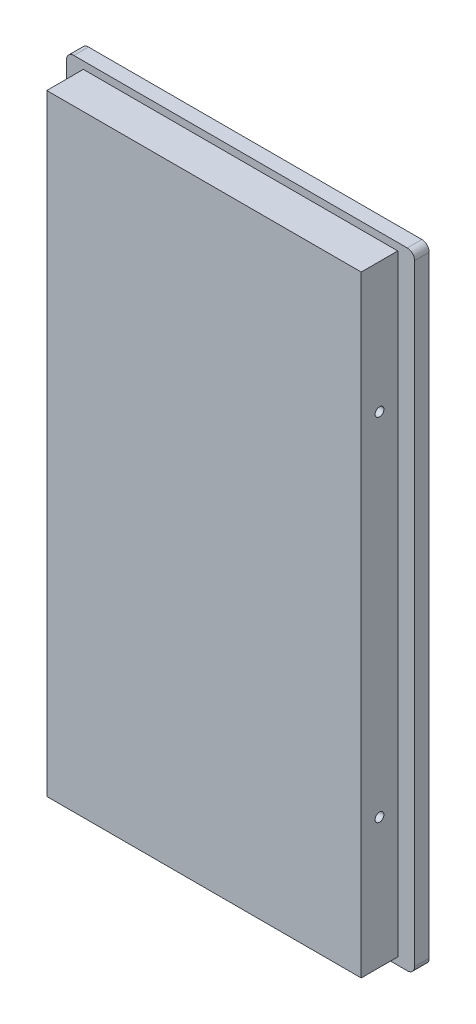
from build123d import *

# Parameters (mm, degrees)
EXTRUDE_1_DEPTH          = 10
SKETCH_2_W               = 215
SKETCH_2_H               = 418
EXTRUDE_2_DEPTH          = 25
CUT_EXTRUDE_1_DEPTH      = 314.565383931
CUT_EXTRUDE_1_DEPTH_BACK = 314.565383931
SKETCH_3_R               = 3
SKETCH_4_R               = 12.5
SKETCH_4_W               = 100
SKETCH_4_H               = 60
CUT_EXTRUDE_2_DEPTH      = 1


with BuildPart() as part:
    # 草图1 → 凸台-拉伸1 (new body)
    with BuildSketch(Plane.XY):
        with BuildLine():
            Line((-114, 214), (114, 214))
            ThreePointArc((114, 214), (117.535533906, 212.535533906), (119, 209))
            Line((119, 209), (119, -209))
            ThreePointArc((119, -209), (117.535533906, -212.535533906), (114, -214))
            Line((114, -214), (-114, -214))
            ThreePointArc((-114, -214), (-117.535533906, -212.535533906), (-119, -209))
            Line((-119, -209), (-119, 209))
            ThreePointArc((-119, 209), (-117.535533906, 212.535533906), (-114, 214))
        make_face()
    extrude(amount=EXTRUDE_1_DEPTH)

    # 草图2 → 凸台-拉伸2 (add)
    with BuildSketch(Plane.XY.offset(10)):
        Rectangle(SKETCH_2_W, SKETCH_2_H)
    extrude(amount=EXTRUDE_2_DEPTH)

    # 草图3 → 切除-拉伸1 (cut, two sides: drawn at the far end of the back side and taken through both)
    with BuildSketch(Plane(origin=(107.5, 0, 0), x_dir=(0, 0, -1), z_dir=(1, 0, 0)).offset(-CUT_EXTRUDE_1_DEPTH_BACK)):
        with Locations(Location((-22.5, 120, 0), (0, 0, 90))):
            Circle(SKETCH_3_R)
        with Locations(Location((-22.5, -120, 0), (0, 0, 90))):
            Circle(SKETCH_3_R)
    extrude(amount=CUT_EXTRUDE_1_DEPTH + CUT_EXTRUDE_1_DEPTH_BACK, mode=Mode.SUBTRACT)

    # 草图4 → 切除-拉伸2 (cut)
    with BuildSketch(Plane(origin=(0, 0, 0), x_dir=(-1, 0, 0), z_dir=(0, 0, -1))):
        with Locations((0, -26)):
            Circle(SKETCH_4_R)
        with Locations((60, -26)):
            Circle(SKETCH_4_R)
        with Locations((60, -86)):
            Circle(SKETCH_4_R)
        with Locations((60, -146)):
            Circle(SKETCH_4_R)
        with Locations((0, -86)):
            Circle(SKETCH_4_R)
        with Locations((0, -146)):
            Circle(SKETCH_4_R)
        with Locations(Location((-60, -146, 0), (0, 0, 180))):
            Circle(SKETCH_4_R)
        with Locations(Location((-60, -86, 0), (0, 0, 180))):
            Circle(SKETCH_4_R)
        with Locations(Location((-60, -26, 0), (0, 0, 180))):
            Circle(SKETCH_4_R)
        with Locations((0, 134)):
            Rectangle(SKETCH_4_W, SKETCH_4_H)
        with BuildLine():
            Line((-12.5, 36), (12.5, 36))
            ThreePointArc((12.5, 36), (14.5, 34), (12.5, 32))
            Line((12.5, 32), (-12.5, 32))
            ThreePointArc((-12.5, 32), (-14.5, 34), (-12.5, 36))
        make_face()
        with BuildLine():
            Line((27.5, 36), (52.5, 36))
            ThreePointArc((52.5, 36), (54.5, 34), (52.5, 32))
            Line((52.5, 32), (27.5, 32))
            ThreePointArc((27.5, 32), (25.5, 34), (27.5, 36))
        make_face()
        with BuildLine():
            Line((-27.5, 36), (-52.5, 36))
            ThreePointArc((-52.5, 36), (-54.5, 34), (-52.5, 32))
            Line((-52.5, 32), (-27.5, 32))
            ThreePointArc((-27.5, 32), (-25.5, 34), (-27.5, 36))
        make_face()
    extrude(amount=-CUT_EXTRUDE_2_DEPTH, mode=Mode.SUBTRACT)


solid = part.part
